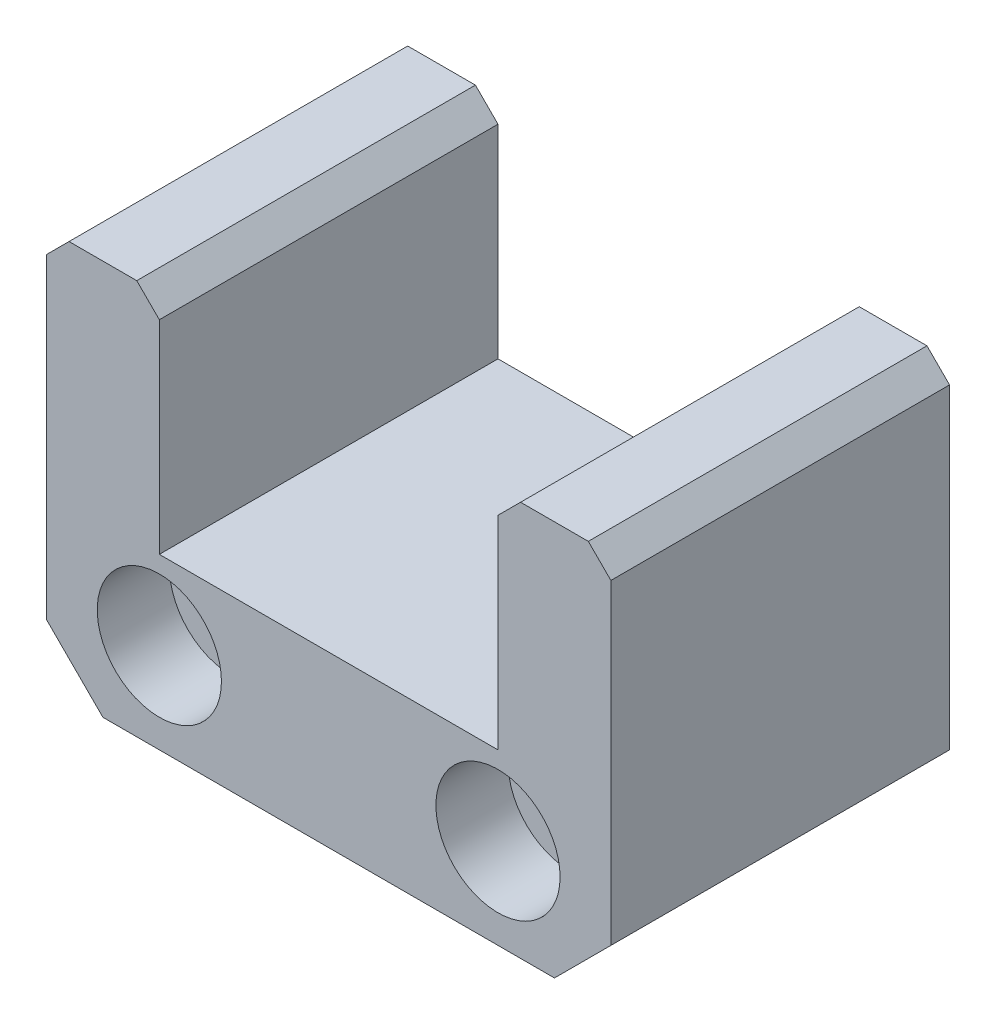
SolidWorks part; units mm, degrees
ref_plane "Front Plane" through (0, 0, 0) normal (0, 0, 1) x (1, 0, 0)
ref_plane "Top Plane" through (0, 0, 0) normal (0, 1, 0) x (1, 0, 0)
ref_plane "Right Plane" through (0, 0, 0) normal (1, 0, 0) x (0, 0, -1)
sketch "Sketch1" plane through (0, 0, 0) normal (0, 0, 1) x (1, 0, 0)
  line L0 (-25, 20) -> (-15, 20)
  line L1 (-15, 20) -> (-15, 0)
  line L2 (-15, 0) -> (15, 0)
  line L3 (15, 0) -> (15, 20)
  line L4 (15, 20) -> (25, 20)
  line L5 (25, 20) -> (25, -15)
  line L6 (25, -15) -> (-25, -15)
  line L7 (-25, -15) -> (-25, 20)
  line L8 (0, 0) -> (0, 66.4423) construction
  dimension "D1" = 30
  dimension "D2" = 50
  dimension "D3" = 20
  dimension "D4" = 35
extrude "Boss-Extrude1" add sketch "Sketch1" along normal blind 30
hole_wizard "CBORE for M6 Hex Socket Head Cap Screw1" positions "Sketch3" profile "Sketch2" counterbore size "M6" standard "Iso" end condition through all
sketch "Sketch3" plane through (0, 0, 30) normal (0, 0, 1) x (1, 0, 0)
  line L0 (0, 0) -> (0, -33.2375) construction
  line L2 (-25, -15) -> (25, -15) construction
  point P0 (-15, -7)
  point P2 (15, -7)
  dimension "D1" = 30
  dimension "D2" = 8
sketch "Sketch2" plane through (-15, -7, 30) normal (1, 0, 0) x (0, -1, 0)
  line L0 (0, 0) -> (0, 30)
  line L1 (0, 30) -> (3.3, 30)
  line L3 (3.3, 30) -> (3.3, 6.4)
  line L4 (3.3, 6.4) -> (5.5, 6.4)
  line L5 (5.5, 6.4) -> (5.5, 0)
  line L7 (5.5, 0) -> (0, 0)
  line L11 (0, -6.35) -> (0, 107.95) construction
  dimension "通孔孔直径" = 6.6
  dimension "通孔孔深度" = 30
  dimension "柱形沉头孔直径" = 11
  dimension "柱形沉头孔深度" = 6.4
chamfer "Chamfer1" distance 2 angle 45 4 edges at (25, 20, 15) (15, 20, 15) (-15, 20, 15) (-25, 20, 15)
chamfer "Chamfer2" distance 5 angle 45 2 edges at (25, -15, 15) (-25, -15, 15)
